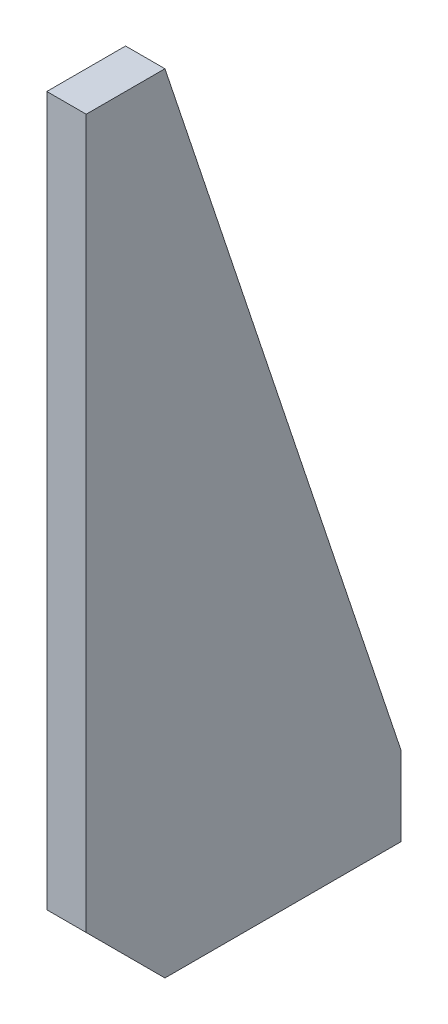
SolidWorks part; units mm, degrees
material "Q235B"
ref_plane "Front Plane" through (0, 0, 0) normal (0, 0, 1) x (1, 0, 0)
ref_plane "Top Plane" through (0, 0, 0) normal (0, 1, 0) x (1, 0, 0)
ref_plane "Right Plane" through (0, 0, 0) normal (1, 0, 0) x (0, 0, -1)
other "Configuration Table"
sketch "Sketch1" plane through (0, 0, 0) normal (1, 0, 0) x (0, 0, -1)
  line L0 (-20, 100) -> (40, -80)
  line L1 (-20, -100) -> (40, -100)
  line L2 (-40, -80) -> (-40, 100)
  line L3 (-40, 100) -> (40, 100)
  line L4 (40, -100) -> (40, 100)
  line L5 (-40, -100) -> (40, 100) construction
  line L6 (-40, 100) -> (40, -100) construction
  line L7 (-40, -80) -> (-20, -100)
  point P0 (0, 0)
  dimension "D1" = 20
  dimension "D2" = 20
  dimension "D3" = 200
  dimension "D4" = 80
extrude "Boss-Extrude1" add sketch "Sketch1" along normal blind 10 contours L2 L7 L1 L4 L0 L3
